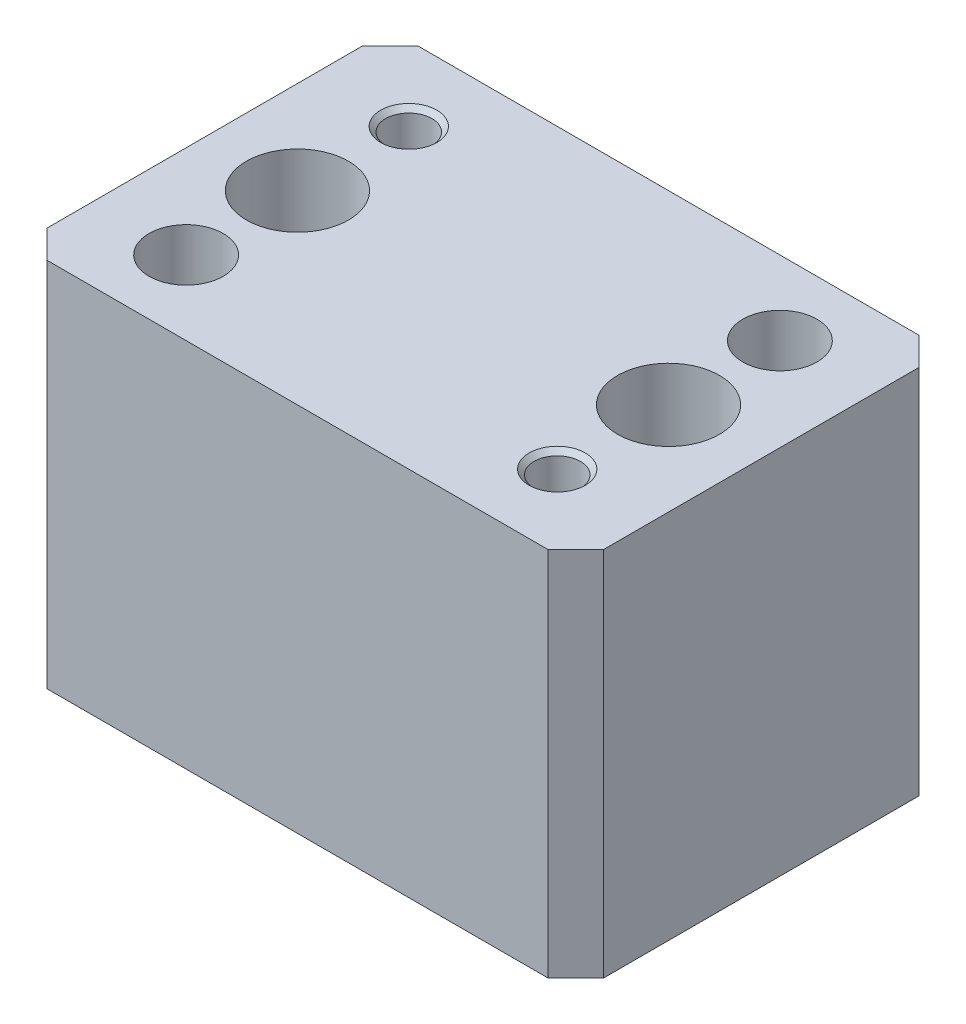
SolidWorks part; units mm, degrees
material "Q235-A"
ref_plane "Front Plane" through (0, 0, 0) normal (0, 0, 1) x (1, 0, 0)
ref_plane "Top Plane" through (0, 0, 0) normal (0, 1, 0) x (1, 0, 0)
ref_plane "Right Plane" through (0, 0, 0) normal (1, 0, 0) x (0, 0, -1)
sketch "Sketch1" plane through (0, 0, 0) normal (0, 0, 1) x (1, 0, 0)
  line L1 (-32.229, 20.7895) -> (27.771, 20.7895)
  line L2 (-32.229, 20.7895) -> (-32.229, -19.2105)
  line L3 (-32.229, -19.2105) -> (27.771, -19.2105)
  line L4 (27.771, 20.7895) -> (27.771, -19.2105)
  dimension "D1" = 60
  dimension "D2" = 40
extrude "Boss-Extrude1" add sketch "Sketch1" along normal blind 40
chamfer "Chamfer1" distance 3 angle 45 4 edges at (27.771, 0.7895, 40) (27.771, 0.7895, 0) (-32.229, 0.7895, 40) (-32.229, 0.7895, 0)
sketch "Sketch2" plane through (0, 20.7895, 0) normal (0, 1, 0) x (1, 0, 0)
  line L0 (27.771, -37) -> (27.771, -3) construction
  line L1 (-22.229, -8) -> (17.771, -8) construction
  line L2 (-22.229, -8) -> (-22.229, -32) construction
  line L3 (-22.229, -32) -> (17.771, -32) construction
  line L4 (17.771, -8) -> (17.771, -32) construction
  line L5 (24.771, -40) -> (-29.229, -40) construction
  line L6 (-22.229, -20) -> (17.771, -20) construction
  dimension "D1" = 40
  dimension "D2" = 24
  dimension "D3" = 10
  dimension "D4" = 8
hole_wizard "M6 Tapped Hole1" positions "Sketch3" profile "Sketch4" tap size "M6" standard "GB"
sketch "Sketch3" plane through (0, 20.7895, 0) normal (0, 1, 0) x (1, 0, 0)
  point P0 (-22.229, -8)
  point P3 (17.771, -32)
sketch "Sketch4" plane through (-22.229, 20.7895, 8) normal (1, 0, 0) x (0, 0, 1)
  line L0 (0, 0) -> (0, 12)
  line L1 (0, 12) -> (2.5, 10.4978)
  line L2 (2.5, 10.4978) -> (2.5, 0.525)
  line L3 (2.5, 0.525) -> (3.025, 0)
  line L5 (3.025, 0) -> (0, 0)
  line L6 (-2.5, 0.525) -> (-3.025, 0) construction
  line L10 (0, 12) -> (-2.5, 10.4978) construction
  line L11 (0, -6.35) -> (0, 107.95) construction
  dimension "螺纹孔钻头直径" = 5
  dimension "螺纹孔钻头深度" = 12
  dimension "近端锥形沉头孔直径" = 6.05
  dimension "近端锥形沉头孔角度" = 90
  dimension "导头角度" = 118
cosmetic thread "Cosmetic thread 1" parameters "D1"=10.4978, "D2"=6
cosmetic thread "Cosmetic thread 2" parameters "D1"=10.4978, "D2"=6
hole_wizard "Hole1" positions "Sketch5" profile "Sketch6" legacy end condition through all
sketch "Sketch5" plane through (0, 20.7895, 0) normal (0, 1, 0) x (1, 0, 0)
  point P0 (-22.229, -20)
  point P3 (17.771, -20)
sketch "Sketch6" plane through (-22.229, 20.7895, 20) normal (1, 0, 0) x (0, 0, 1)
  line L0 (0, 0) -> (0, 40)
  line L1 (0, 40) -> (3.3, 40)
  line L2 (3.3, 40) -> (3.3, 27)
  line L3 (3.3, 27) -> (5.5, 27)
  line L4 (5.5, 27) -> (5.5, 0)
  line L5 (5.5, 0) -> (0, 0)
  line L6 (0, 110) -> (0, -10) construction
  dimension "直径" = 6.6
  dimension "深度" = 40
  dimension "柱坑直径" = 11
  dimension "柱坑深度" = 27
hole_wizard "Hole2" positions "Sketch7" profile "Sketch8" legacy
sketch "Sketch7" plane through (0, 20.7895, 0) normal (0, 1, 0) x (1, 0, 0)
  point P0 (17.771, -8)
  point P3 (-22.229, -32)
sketch "Sketch8" plane through (17.771, 20.7895, 8) normal (1, 0, 0) x (0, 0, 1)
  line L0 (0, 0) -> (0, 9)
  line L1 (0, 9) -> (4, 9)
  line L2 (4, 9) -> (4, 0)
  line L3 (4, 0) -> (0, 0)
  line L4 (0, 110) -> (0, -10) construction
  dimension "直径" = 8
  dimension "深度" = 9
sketch "Sketch9" plane through (0, -19.2105, 0) normal (0, -1, 0) x (1, 0, 0)
  line L0 (-2.229, 34) -> (-2.229, 6)
  line L1 (-22.229, 20) -> (17.771, 20) construction
  point P2 (-2.229, 20)
  dimension "D1" = 28
hole_wizard "Hole3" positions "Sketch10" profile "Sketch11" legacy
sketch "Sketch10" plane through (0, -19.2105, 0) normal (0, -1, 0) x (-1, 0, 0)
  point P0 (2.229, -34)
  point P3 (2.229, -6)
sketch "Sketch11" plane through (-2.229, -19.2105, 34) normal (1, 0, 0) x (0, 0, -1)
  line L0 (0, 0) -> (0, 8.5)
  line L1 (0, 8.5) -> (4, 8.5)
  line L2 (4, 8.5) -> (4, 0)
  line L3 (4, 0) -> (0, 0)
  line L4 (0, 110) -> (0, -10) construction
  dimension "直径" = 8
  dimension "深度" = 8.5
